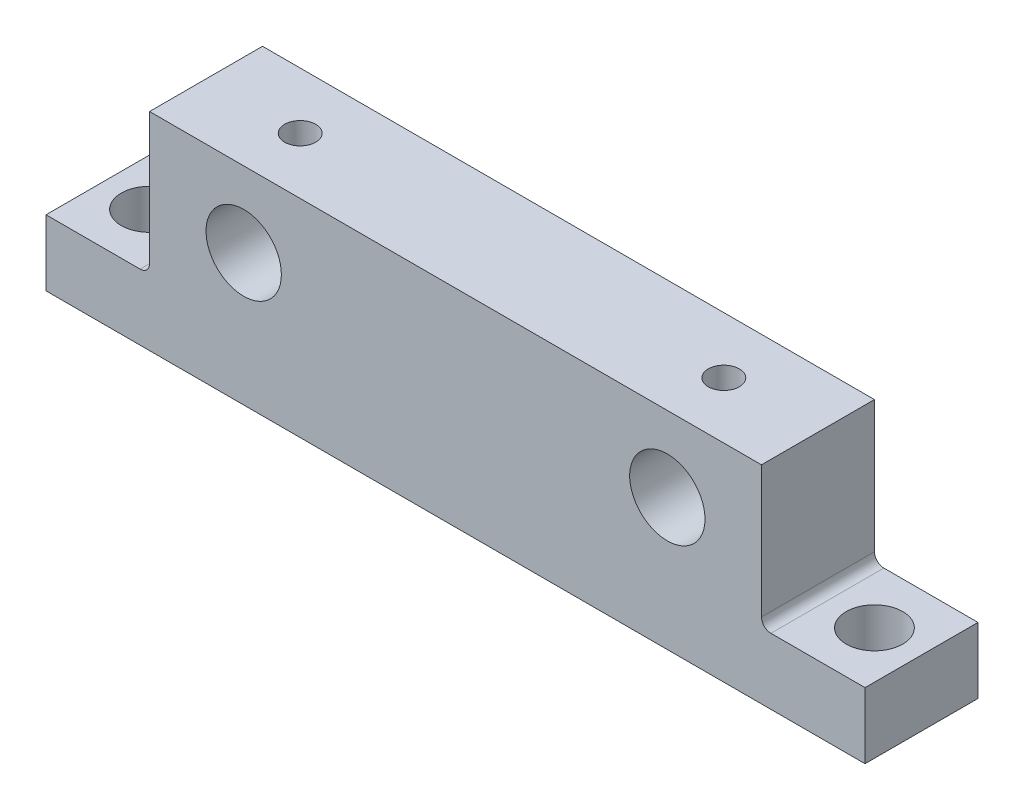
from build123d import *

# Parameters (mm, degrees)
SKETCH_1_R              = 4
EXTRUDE_1_DEPTH         = 6
HOLE_WIZARD_M4_1_REACH  = 71.828
HOLE_WIZARD_M4_1_BORE_R = 1.65
FILLET_1_R              = 1
CUT_EXTRUDE_1_REACH     = 48.403
SKETCH_3_R              = 3


with BuildPart() as part:
    # 草图1 → 凸台-拉伸1 (new, symmetric)
    with BuildSketch(Plane.XY):
        Polygon((0, 0), (-32.5, 0), (-32.5, -15), (-43.5, -15), (-43.5, -22), (43.5, -22), (43.5, -15), (32.5, -15), (32.5, 0), align=None)
        with Locations((-22.5, -8)):
            Circle(SKETCH_1_R, mode=Mode.SUBTRACT)
        with Locations((22.5, -8)):
            Circle(SKETCH_1_R, mode=Mode.SUBTRACT)
    extrude(amount=EXTRUDE_1_DEPTH, both=True)

    # M4 螺纹孔1 bore (on position points) → M4 螺纹孔1 (cut, up to next)
    with BuildSketch(Plane(origin=(-22.5, 0, 0), x_dir=(1, 0, 0), z_dir=(0, 1, 0)), mode=Mode.PRIVATE) as hole_wizard_m4_1_sk1:
        Circle(HOLE_WIZARD_M4_1_BORE_R)
    hole_wizard_m4_1_tool1 = extrude(hole_wizard_m4_1_sk1.sketch, amount=-HOLE_WIZARD_M4_1_REACH, mode=Mode.PRIVATE) & part.part
    hole_wizard_m4_1 = hole_wizard_m4_1_tool1.solids().sort_by_distance((-22.5, 0, 0))[0]
    add(hole_wizard_m4_1, mode=Mode.SUBTRACT)

    # 镜向1: M4 螺纹孔1 across plane
    add(hole_wizard_m4_1.mirror(Plane(origin=(0, 0, 0), x_dir=(0, 0, 1), z_dir=(1, 0, 0))), mode=Mode.SUBTRACT)

    # 圆角1
    fillet_1_edges = [part.edges().sort_by_distance(p)[0] for p in [
        (32.5, -15, 0),
        (-32.5, -15, 0),
    ]]
    fillet(fillet_1_edges, radius=FILLET_1_R)

    # 草图3 → 切除-拉伸1 (cut, up to next)
    with BuildSketch(Plane(origin=(0, -15, 0), x_dir=(1, 0, 0), z_dir=(0, 1, 0)), mode=Mode.PRIVATE) as cut_extrude_1_sk1:
        with Locations(Location((-38.5, 0, 0), (0, 0, 270))):
            Circle(SKETCH_3_R)
    cut_extrude_1_tool1 = extrude(cut_extrude_1_sk1.sketch, amount=-CUT_EXTRUDE_1_REACH, mode=Mode.PRIVATE) & part.part
    # 草图3 → 切除-拉伸1 (cut, up to next)
    with BuildSketch(Plane(origin=(0, -15, 0), x_dir=(1, 0, 0), z_dir=(0, 1, 0)), mode=Mode.PRIVATE) as cut_extrude_1_sk2:
        with Locations(Location((38.5, 0, 0), (0, 0, 270))):
            Circle(SKETCH_3_R)
    cut_extrude_1_tool2 = extrude(cut_extrude_1_sk2.sketch, amount=-CUT_EXTRUDE_1_REACH, mode=Mode.PRIVATE) & part.part
    add(cut_extrude_1_tool1.solids().sort_by_distance((-38.5, -15, 0))[0], mode=Mode.SUBTRACT)
    add(cut_extrude_1_tool2.solids().sort_by_distance((38.5, -15, 0))[0], mode=Mode.SUBTRACT)


solid = part.part
